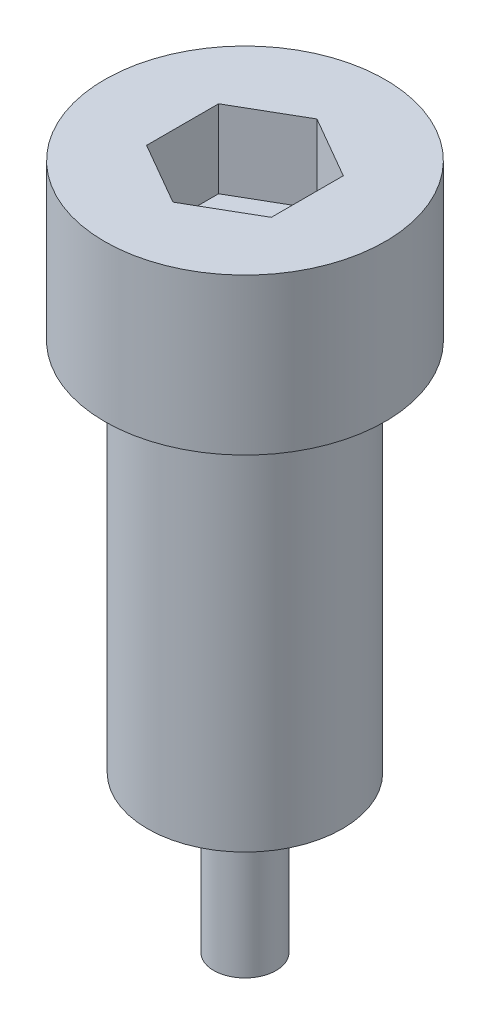
SolidWorks part; units mm, degrees
material "45"
ref_plane "Front Plane" through (0, 0, 0) normal (0, 0, 1) x (1, 0, 0)
ref_plane "Top Plane" through (0, 0, 0) normal (0, 1, 0) x (1, 0, 0)
ref_plane "Right Plane" through (0, 0, 0) normal (1, 0, 0) x (0, 0, -1)
sketch "Sketch1" plane through (0, 0, 0) normal (0, 1, 0) x (1, 0, 0)
  circle A0 centre (0, 0) radius 2
  dimension "D1" = 4
extrude "Boss-Extrude1" add sketch "Sketch1" along normal blind 10
cosmetic thread "Cosmetic Thread1" parameters "D2"=3.242
sketch "Sketch2" plane through (0, 10, 0) normal (0, 1, 0) x (1, 0, 0)
  circle A0 centre (0, 0) radius 6.25
  dimension "D1" = 12.5
extrude "Boss-Extrude2" add sketch "Sketch2" along normal blind 24
sketch "Sketch3" plane through (0, 34, 0) normal (0, 1, 0) x (1, 0, 0)
  circle A0 centre (0, 0) radius 9
  dimension "D1" = 18
extrude "Boss-Extrude3" add sketch "Sketch3" along normal blind 10
sketch "Sketch4" plane through (0, 44, 0) normal (0, 1, 0) x (1, 0, 0)
  line L1 (0, 4.6188) -> (-4, 2.3094)
  line L2 (-4, 2.3094) -> (-4, -2.3094)
  line L3 (-4, -2.3094) -> (0, -4.6188)
  line L4 (0, -4.6188) -> (4, -2.3094)
  line L5 (4, -2.3094) -> (4, 2.3094)
  line L6 (4, 2.3094) -> (0, 4.6188)
  circle A0 centre (0, 0) radius 4 construction
  dimension "D2" = 8
extrude "Cut-Extrude1" cut sketch "Sketch4" against normal blind 5
